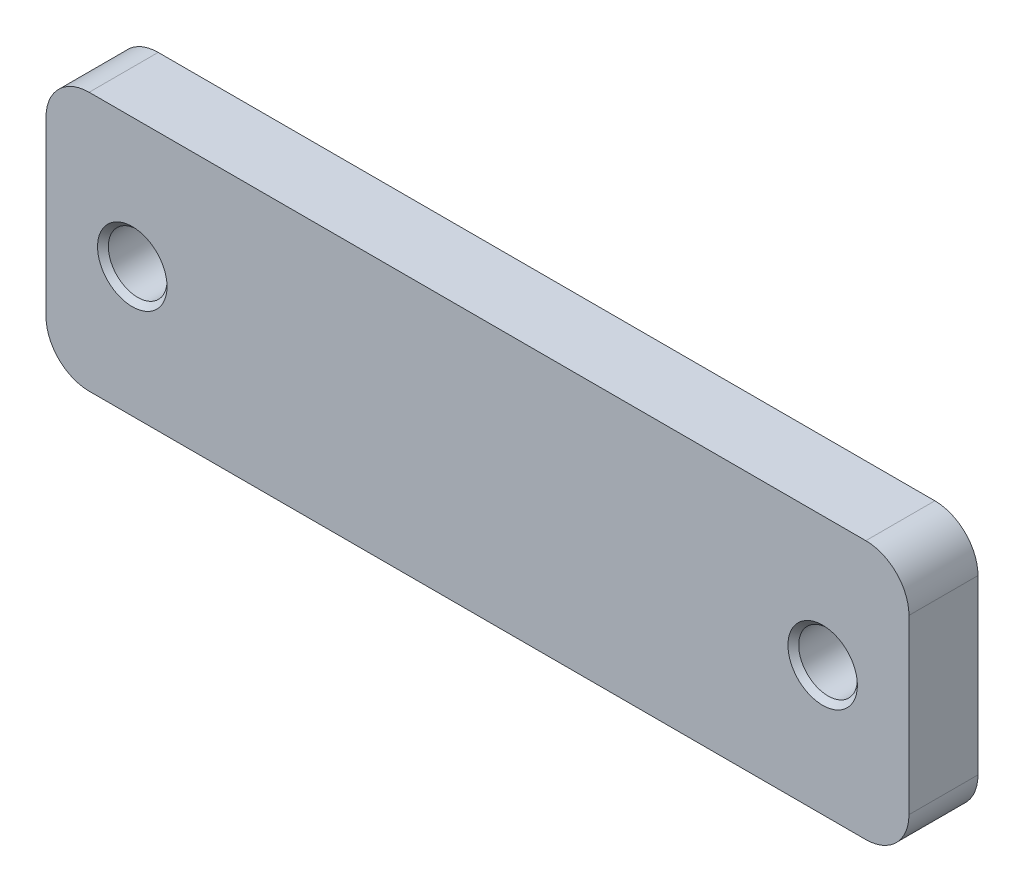
SolidWorks part; units mm, degrees
ref_plane "Front Plane" through (0, 0, 0) normal (0, 0, 1) x (1, 0, 0)
ref_plane "Top Plane" through (0, 0, 0) normal (0, 1, 0) x (1, 0, 0)
ref_plane "Right Plane" through (0, 0, 0) normal (1, 0, 0) x (0, 0, -1)
other "Configuration Table"
sketch "Sketch1" plane through (0, 0, 0) normal (0, 0, 1) x (1, 0, 0)
  line L1 (-50, -15) -> (50, -15)
  line L2 (-50, -15) -> (-50, 15)
  line L3 (-50, 15) -> (50, 15)
  line L4 (50, -15) -> (50, 15)
  line L5 (-50, -15) -> (50, 15) construction
  line L6 (-50, 15) -> (50, -15) construction
  point P0 (0, 0)
  dimension "D1" = 100
  dimension "D2" = 30
extrude "Boss-Extrude1" add sketch "Sketch1" along normal blind 8
fillet "Fillet1" radius 5 4 edges at (50, -15, 4) (50, 15, 4) (-50, -15, 4) (-50, 15, 4)
hole_wizard "M8 Tapped Hole1" positions "Sketch2" profile "Sketch3" tap size "M8" standard "GB" end condition through all
sketch "Sketch2" plane through (0, 0, 8) normal (0, 0, 1) x (1, 0, 0)
  line L0 (-50, 10) -> (-50, -10) construction
  line L1 (50, -10) -> (50, 10) construction
  line L2 (-50, 0) -> (50, 0) construction
  point P0 (-40, 0)
  point P2 (40, 0)
  dimension "D1" = 10
  dimension "D2" = 10
sketch "Sketch3" plane through (-40, 0, 8) normal (1, 0, 0) x (0, -1, 0)
  line L0 (0, 0) -> (0, 8)
  line L1 (0, 8) -> (3.4, 8)
  line L2 (3.4, 8) -> (3.4, 0.625)
  line L3 (3.4, 0.625) -> (4.025, 0)
  line L5 (4.025, 0) -> (0, 0)
  line L6 (-3.4, 0.625) -> (-4.025, 0) construction
  line L11 (0, -6.35) -> (0, 107.95) construction
  dimension "通孔螺纹孔钻头直径" = 6.8
  dimension "通孔螺纹孔钻头深度" = 8
  dimension "近端锥形沉头孔直径" = 8.05
  dimension "近端锥形沉头孔角度" = 90
cosmetic thread "Cosmetic Thread 1" parameters "D2"=8
cosmetic thread "Cosmetic Thread 2" parameters "D2"=8
